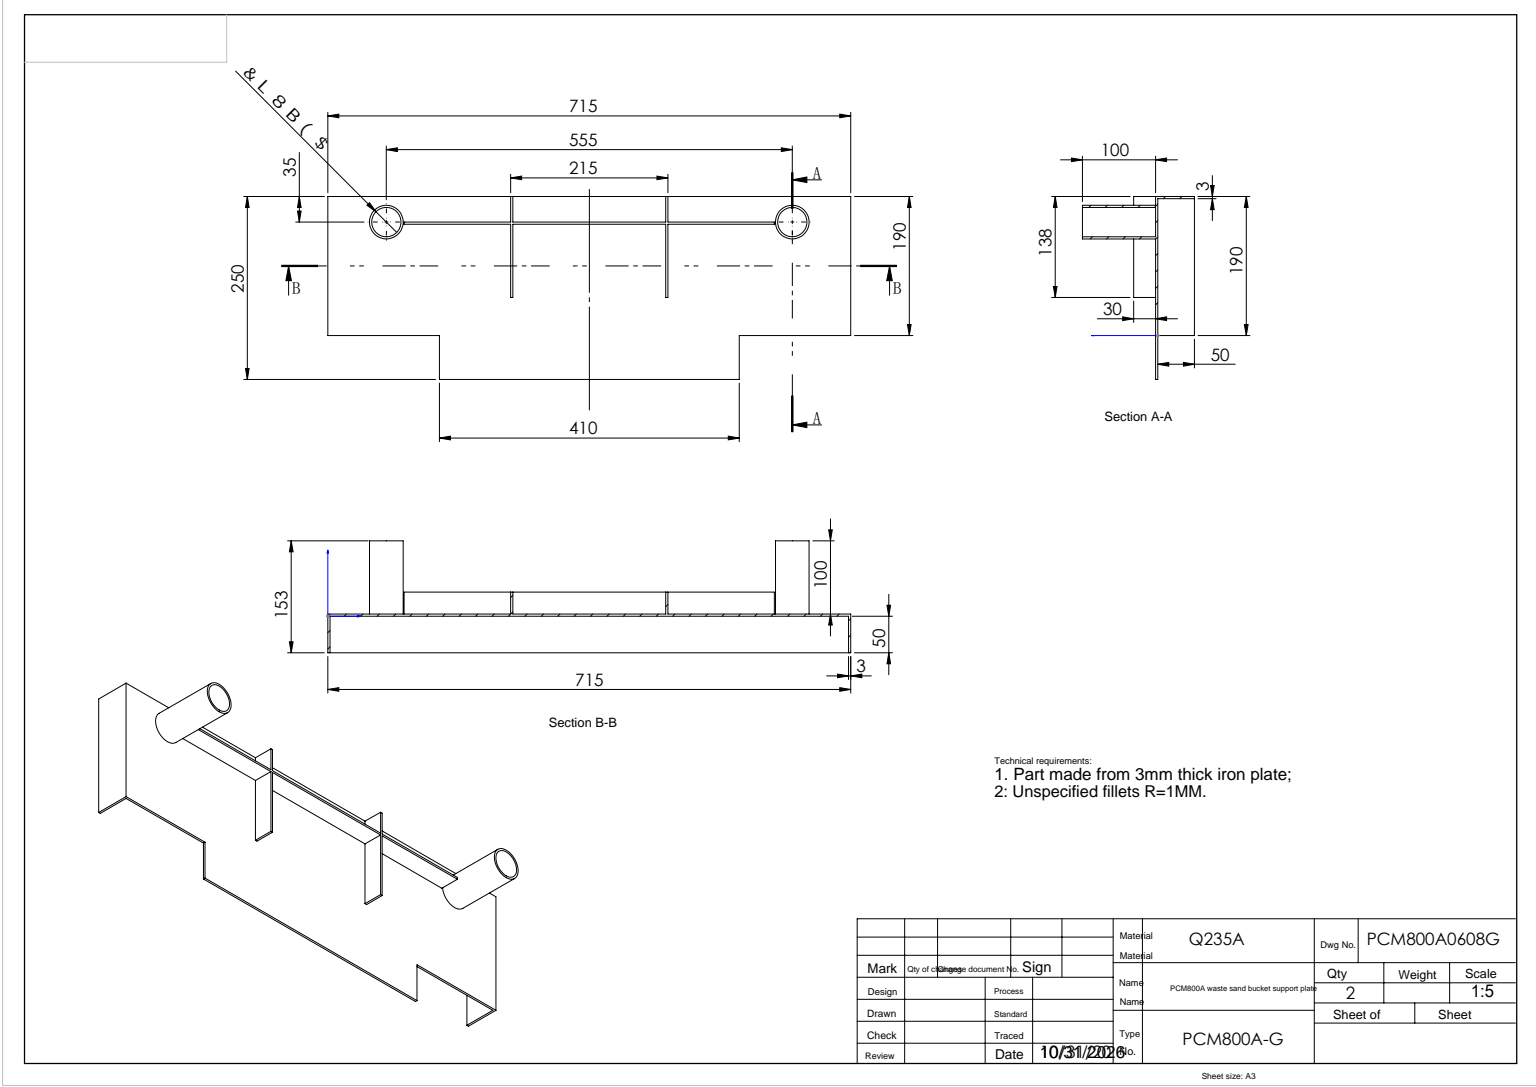
SolidWorks part; units mm, degrees
ref_plane "前视" through (0, 0, 0) normal (0, 0, 1) x (1, 0, 0)
ref_plane "上视" through (0, 0, 0) normal (0, 1, 0) x (1, 0, 0)
ref_plane "右视" through (0, 0, 0) normal (1, 0, 0) x (0, 0, -1)
sketch "草图1" plane through (0, 0, 0) normal (0, 1, 0) x (1, 0, 0)
  line L0 (357.5, 190) -> (357.5, -60) construction
  line L1 (357.5, -60) -> (152.5, -60)
  line L2 (0, 0) -> (0, 190)
  line L3 (0, 190) -> (715, 190)
  line L4 (715, 0) -> (715, 190)
  line L5 (357.5, -60) -> (562.5, -60)
  line L6 (152.5, -60) -> (152.5, 0)
  line L7 (152.5, 0) -> (0, 0)
  line L8 (562.5, -60) -> (562.5, 0)
  line L9 (562.5, 0) -> (715, 0)
  dimension "D1" = 190
  dimension "D2" = 715
  dimension "D3" = 205
  dimension "D4" = 205
  dimension "D5" = 250
  dimension "D6" = 190
extrude "凸台-拉伸1" add sketch "草图1" along normal blind 3
sketch "草图2" plane through (0, 3, 0) normal (0, 1, 0) x (1, 0, 0)
  line L0 (715, 190) -> (0, 190) construction
  line L1 (80, 155) -> (728.8983, 155) construction
  line L2 (0, 190) -> (0, 0) construction
  line L3 (715, 0) -> (715, 190) construction
  circle A0 centre (80, 155) radius 20
  circle A1 centre (635, 155) radius 20
  circle A2 centre (80, 155) radius 23
  circle A3 centre (635, 155) radius 23
  dimension "D1" = 40
  dimension "D2" = 40
  dimension "D3" = 35
  dimension "D4" = 80
  dimension "D5" = 80
extrude "凸台-拉伸2" add sketch "草图2" along normal blind 100
sketch "草图4" plane through (715, 0, 0) normal (1, 0, 0) x (0, 0, -1)
  line L1 (190, 0) -> (187, 0)
  line L2 (190, 0) -> (190, -50)
  line L3 (190, -50) -> (187, -50)
  line L4 (187, 0) -> (187, -50)
  dimension "D1" = 3
  dimension "D2" = 50
extrude "凸台-拉伸3" add sketch "草图4" against normal up to surface (715 mm away) separate body up to face at (0, 1.5, -95)
sketch "草图7" plane through (0, 3, 0) normal (0, 1, 0) x (1, 0, 0)
  line L0 (80, 155) -> (635, 155) construction
  line L2 (104.2239, 155) -> (610.5389, 155)
  line L3 (104.2239, 155) -> (104.2239, 152)
  line L4 (104.2239, 152) -> (610.5389, 152)
  line L5 (610.5389, 155) -> (610.5389, 152)
  dimension "D1" = 3
extrude "凸台-拉伸8" add sketch "草图7" along normal blind 30
sketch "草图8" plane through (0, 3, 0) normal (0, 1, 0) x (1, 0, 0)
  line L0 (610.5389, 155) -> (104.2239, 155) construction
  line L1 (250, 155) -> (253, 155)
  line L2 (250, 155) -> (250, 190)
  line L3 (250, 190) -> (253, 190)
  line L4 (253, 155) -> (253, 190)
  line L5 (715, 190) -> (0, 190) construction
  line L6 (104.2239, 152) -> (610.5389, 152) construction
  line L7 (250, 152) -> (253, 152)
  line L8 (250, 152) -> (250, 52)
  line L9 (250, 52) -> (253, 52)
  line L10 (253, 152) -> (253, 52)
  line L11 (357.5, -60) -> (357.5, 301.5529) construction
  line L12 (152.5, -60) -> (562.5, -60) construction
  line L13 (0, 190) -> (0, 0) construction
  line L14 (462, 152) -> (462, 52)
  line L15 (465, 52) -> (462, 52)
  line L16 (465, 152) -> (465, 52)
  line L17 (465, 152) -> (462, 152)
  line L18 (462, 155) -> (462, 190)
  line L19 (465, 190) -> (462, 190)
  line L20 (465, 155) -> (465, 190)
  line L21 (465, 155) -> (462, 155)
  dimension "D1" = 3
  dimension "D2" = 250
  dimension "D3" = 250
  dimension "D4" = 3
  dimension "D5" = 100
extrude "凸台-拉伸9" add sketch "草图8" along normal blind 30
sketch "草图9" plane through (0, 0, 0) normal (0, 0, 1) x (1, 0, 0)
  line L0 (0, -50) -> (715, -50) construction
  line L1 (715, 0) -> (712, 0)
  line L2 (715, 0) -> (715, -50)
  line L3 (715, -50) -> (712, -50)
  line L4 (712, 0) -> (712, -50)
  line L5 (357.5, 33) -> (357.5, -121.4103) construction
  line L6 (253, 33) -> (462, 33) construction
  line L7 (3, 0) -> (3, -50)
  line L8 (0, -50) -> (3, -50)
  line L9 (0, 0) -> (0, -50)
  line L10 (0, 0) -> (3, 0)
  dimension "D1" = 3
extrude "凸台-拉伸10" add sketch "草图9" against normal up to surface (187 mm away) up to face at (357.5, -25, -187)
